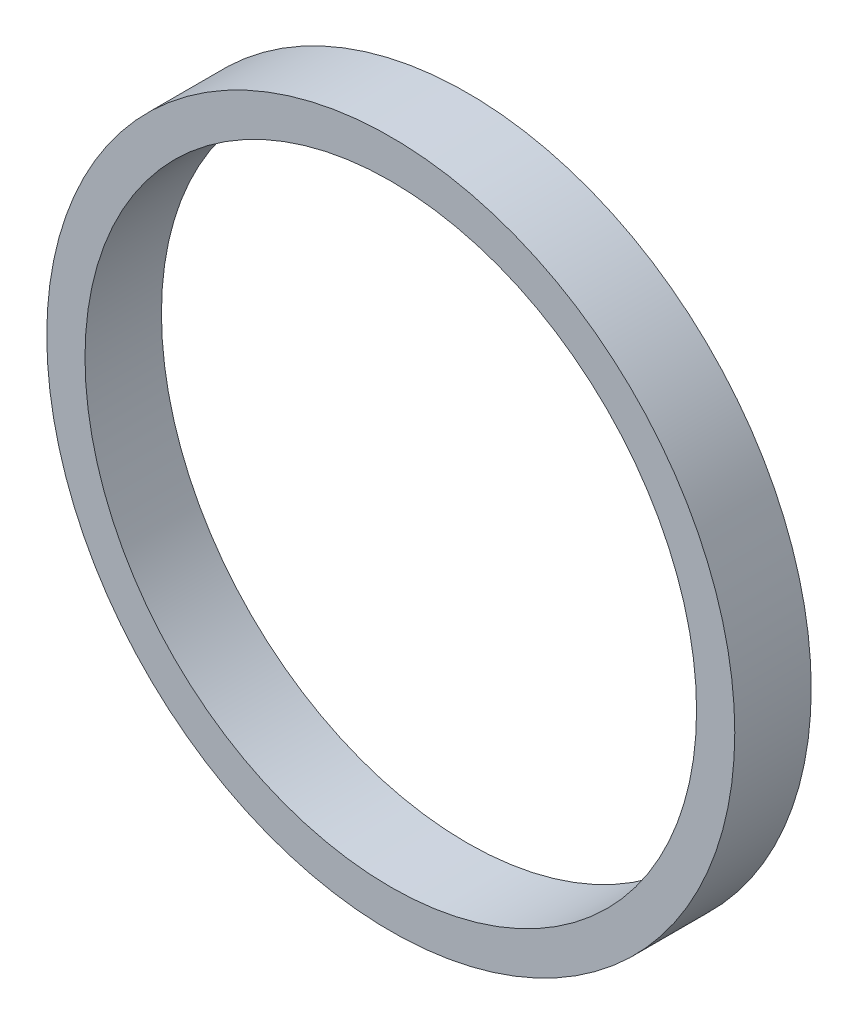
from build123d import *

# Parameters (mm, degrees)
SKETCH1_R           = 4.5
SKETCH1_R_2         = 4
BOSS_EXTRUDE1_DEPTH = 1


with BuildPart() as part:
    # Sketch1 → Boss-Extrude1 (new body)
    with BuildSketch(Plane.XY):
        Circle(SKETCH1_R)
        Circle(SKETCH1_R_2, mode=Mode.SUBTRACT)
    extrude(amount=BOSS_EXTRUDE1_DEPTH)


solid = part.part
